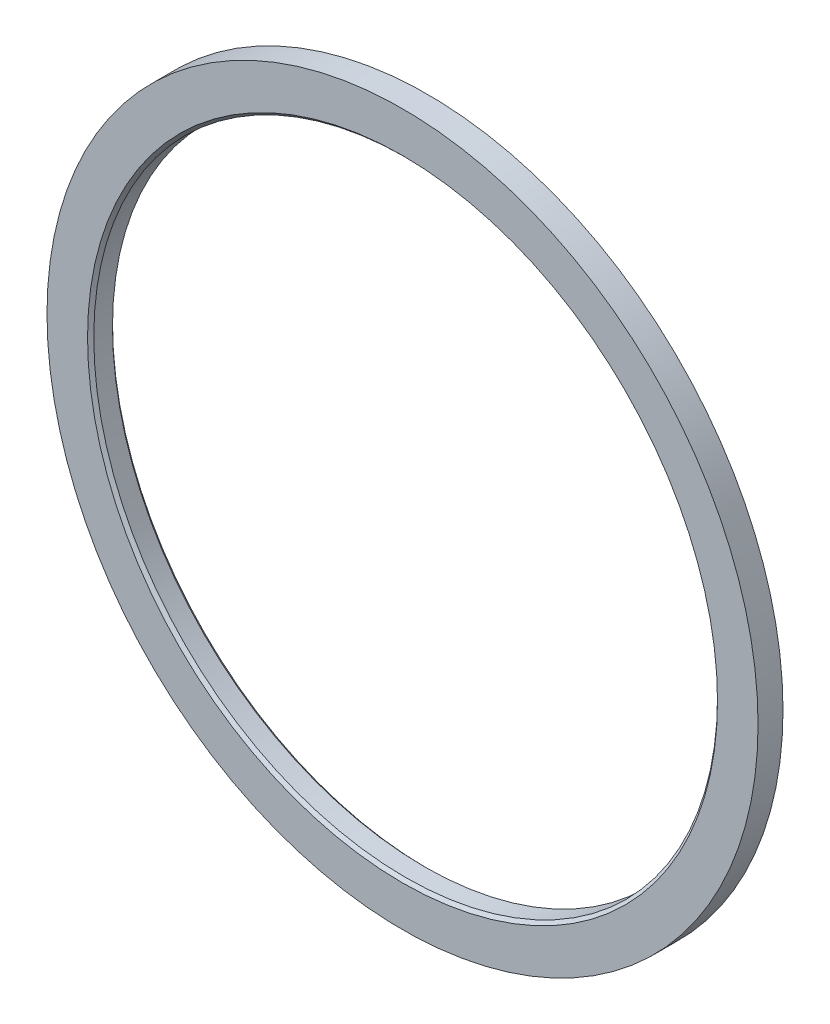
SolidWorks part; units mm, degrees
ref_plane "Front Plane" through (0, 0, 0) normal (0, 0, 1) x (1, 0, 0)
ref_plane "Top Plane" through (0, 0, 0) normal (0, 1, 0) x (1, 0, 0)
ref_plane "Right Plane" through (0, 0, 0) normal (1, 0, 0) x (0, 0, -1)
ref_plane "Plane1" through (0, 234.744, 0) normal (0, 1, 0) x (1, 0, 0)
sketch "Sketch1" plane through (0, 234.744, 0) normal (0, 1, 0) x (1, 0, 0)
  line L0 (571.2306, 185.193) -> (571.7306, 184.693)
  line L1 (571.7306, 184.693) -> (578.2306, 184.693)
  line L2 (578.2306, 184.693) -> (578.2306, 188.693)
  line L3 (578.2306, 188.693) -> (571.7306, 188.693)
  line L4 (571.7306, 188.693) -> (571.2306, 188.193)
  line L5 (571.2306, 188.193) -> (571.2306, 185.193)
  line L6 (521.2306, 188.693) -> (521.2306, 184.693) construction
  dimension "D1" = 50
  dimension "D2" = 50.5
  dimension "D3" = 57
  dimension "D4" = 0.5
  dimension "D5" = 3.5
  dimension "D6" = 4
revolve "Revolve1" add sketch "Sketch1" angle 360 about L6
